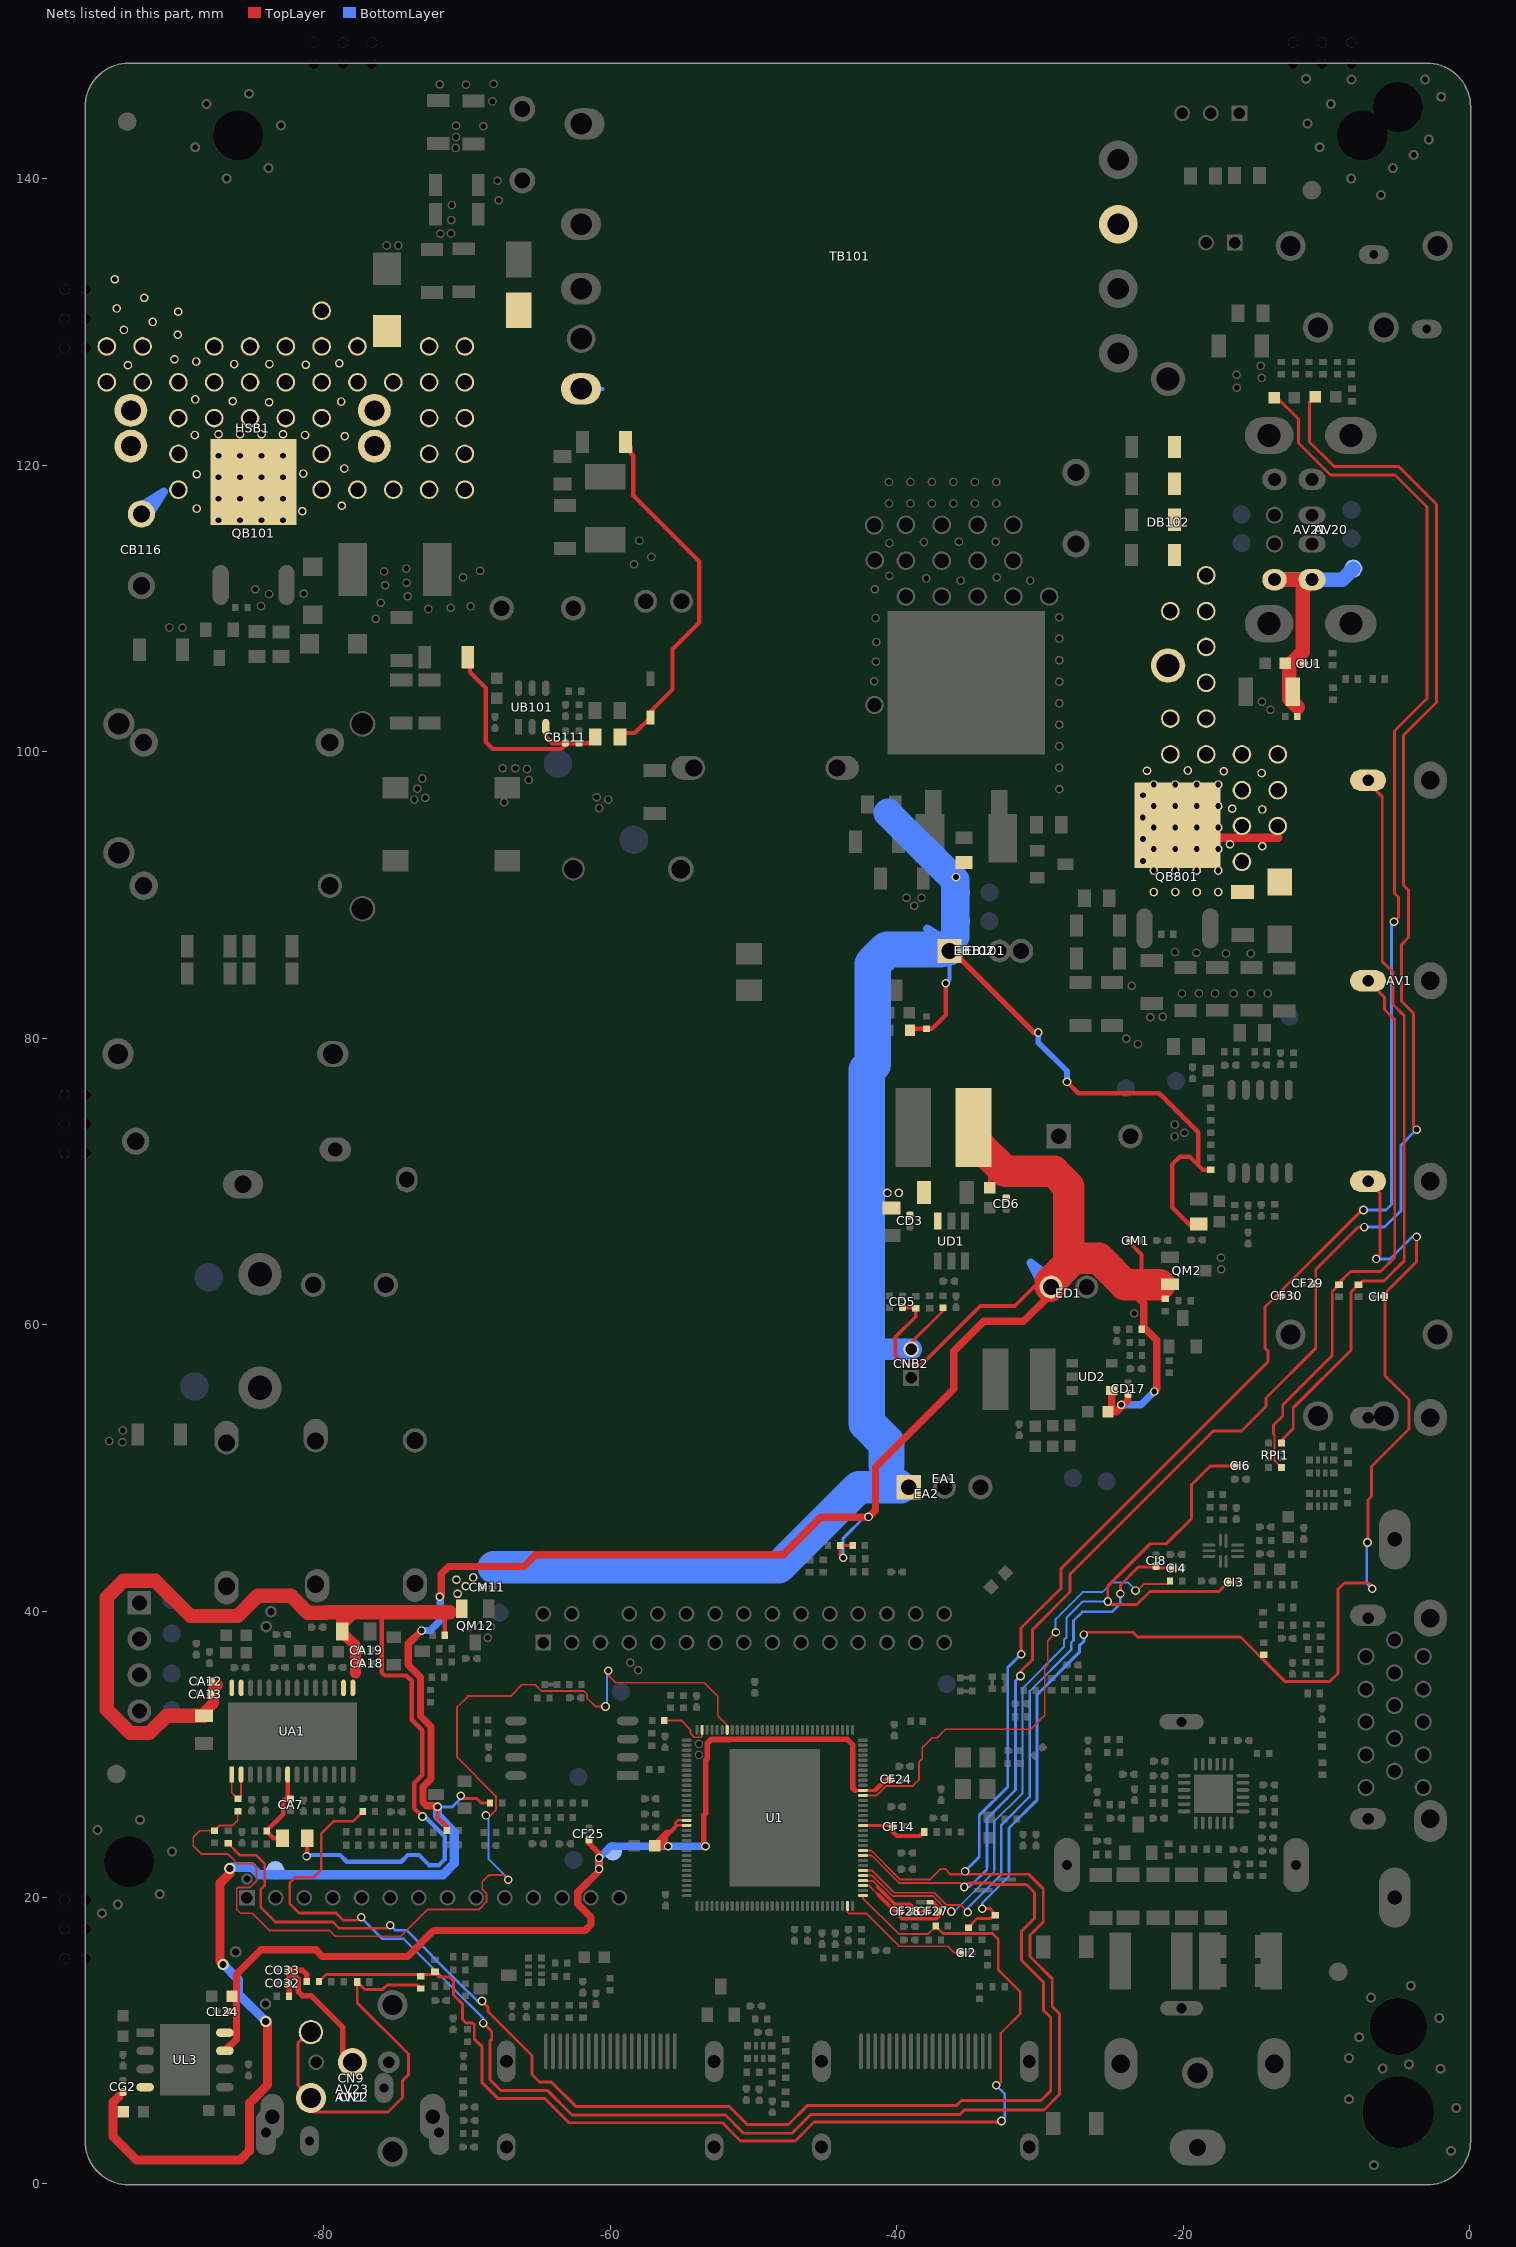
[diagram p0: the nets of this part, all layers, seen from the top]
# Altium PCB MISC86372.PcbDoc (part 7 of 16)
Units mm, origin at the board's own origin, x right, y up, seen from the top; angles counter-clockwise.
Board outline 96.73 x 148.13 mm, 2 copper layers (TopLayer, BottomLayer), stack 1.571 mm thick; 578 components, 318 nets, 2702 pads, 836 vias.

## Via types
v1: diameter 0.6, hole 0.4, TopLayer to BottomLayer, tented both sides, 816 vias
v2: diameter 0.7, hole 0.5, TopLayer to BottomLayer, tented both sides, 15 vias
v3: diameter 0.8, hole 0.5, TopLayer to BottomLayer, tented both sides, 5 vias

## Nets (pads, with @x,y where several pads share a name; then routed paths per layer and width w, separated by ;. In a path a pad name is that pad's centre, name@x,y a point inside that pad or via, vN(x,y) a via of type N, cw(c..) or ccw(c..) an arc to the next point about the centre after c; other vN are vias at no path point) (continued)
5V_STB: 5V_STB.1 CD5.2@-39.603,61.164 CD5.2@-39.603,61.339 CD6.2@-32.36,68.87 CD6.2@-32.36,68.695 CD7.2 CD16.2 CD17.2@-23.849,55.1 CD17.2@-23.849,55.275 CG1.2 CG2.2@-94.027,6.377 CG2.2@-94.027,6.552 CM1.2@-23.556,65.863 CM1.2@-23.731,65.863 ED1.1 LD1.2 pad.VIA5@-22.022,55.321 pad.VIA5@-24.337,54.392 pad.VIA5@-71.907,40.996 pad.VIA5@-73.177,38.633 pad.VIA5@-84.051,11.354 pad.VIA5@-86.563,22.022 pad.VIA5@-87.027,15.327 QM2.S RD3.2 RD7.2 RF8.2 RF9.2 RK1.2 RK5.1 RM3.2 UD2.4 UL3.4 | length 202.9
  TopLayer w0.203: v1(-70.434,27.102) v1@-70.258,26.925 ; v1@-70.423,26.925 v1@-70.258,26.925 ; RK1.2@-68.503,26.702 RK1.2@-68.395,26.594 -69.005,26.594 -69.337,26.925 v1@-70.258,26.925 ; v1(-43.741,43.715) -43.949,43.923 RF9.2@-43.949,44.564 RF8.2@-43.072,44.564
  TopLayer w0.254: CD5.2@-39.603,61.164 -38.702,61.164 RD3.2@-38.677,61.139 -38.677,60.545 -40.083,59.139 -40.083,57.826 -39.449,57.191 -38.268,57.191 -34.168,61.29 -31.766,61.29 -30.372,62.684 ED1.1@-29.293,62.684 ; CD7.2@-33.503,69.551 -33.503,70.841 ; CM1.2@-23.731,65.863 -23.731,65.706 -22.918,64.893 -22.918,62.789
  TopLayer w0.305: v1(-72.063,26.338) -72.063,25.577 -71.418,24.932 RK5.1@-71.418,24.669
  TopLayer w0.381: -23.849,54.736 CD17.2@-23.849,55.1
  TopLayer w0.508: pad.VIA5@-73.177,38.633 -74.1,37.711 -74.1,36.228 -73.254,35.382 -73.254,32.664 -72.517,31.928 -72.517,28.296 ; -73,27.813 -72.517,28.296 ; v1(-72.063,26.338) -72.135,26.41 -72.835,26.41 -73.068,26.643 -73.068,27.738 -72.517,28.289 -72.517,28.296 ; pad.VIA5@-71.797,40.996 -71.797,42.59 -71.283,43.104 -66.026,43.104 -65.197,43.933 -47.916,43.933 -45.3,46.549 -41.973,46.549 -41.478,47.044 -41.478,50.037 -36.018,55.497 -36.018,58.14 -33.934,60.223 -31.153,60.223 -29.293,62.084 ED1.1@-29.293,62.684 ; UD2.4@-24.99,55.393 -24.99,54.015 -25.102,53.904 -24.682,53.904 -23.849,54.736 ; -24.067,62.789 -22.766,61.488 -22.766,59.816 -21.844,58.894 -21.844,55.499 pad.VIA5@-22.022,55.321 ; -21.858,62.569 -21.638,62.789
  TopLayer w0.635: -94.289,6.121 -94.704,5.706 -94.704,3.309 -93.083,1.688 -88.4,1.688 -88.388,1.676 -85.827,1.676 -85.194,2.309 -85.194,5.635 -84.903,5.927 -84.903,5.932 -83.922,6.913 -83.922,11.225 pad.VIA5@-84.051,11.354 ; pad.VIA5@-87.027,15.327 -87.244,15.544 -87.244,20.993 -86.563,21.674 pad.VIA5@-86.563,22.022
  TopLayer w2.2: LD1.2@-34.154,72.425 -32.417,70.688 -29.056,70.688 -27.983,69.615 -27.983,64.263 ; ED1.1@-29.293,62.684 -29.293,62.953 -27.983,64.263 ; -21.638,62.789 -22.918,62.789 -24.067,62.789 -25.899,64.621 -27.625,64.621 -27.983,64.263
  BottomLayer w0.203: v1(-72.063,26.338) -72.037,26.313 -71.036,26.313 v1@-70.423,26.925 ; v1(-43.741,43.715) -43.741,45.082 -42.254,46.569 v1(-41.973,46.569)
  BottomLayer w0.508: pad.VIA5@-73.177,38.633 -72.568,38.633 -71.861,39.341 -71.861,40.996 pad.VIA5@-71.857,40.996 ; ED1.1@-29.228,62.619 ED1.1@-29.228,63.239 ; pad.VIA5@-24.337,54.392 -22.951,54.392 pad.VIA5@-22.022,55.321
  BottomLayer w0.635: pad.VIA5@-87.027,15.327 -85.954,14.254 -85.954,13.257 pad.VIA5@-84.051,11.354 ; pad.VIA5@-86.563,22.022 -86.476,22.109 -85.025,22.109 -84.506,21.59 -71.679,21.59 -70.891,22.377 -70.891,24.551 -72.063,25.723 v1(-72.063,26.338)
5V_USB2.0: 5V.1 AV20.1@-11.01,112 AV21.1 AV21.5 CU1.1 CU2.1 FU1.1 RU4.1 | length 18.3
  TopLayer w1.016: AV21.1@-13.63,112 AV21.5@-11.01,112 -11.665,111.345 -11.665,106.979 -12.598,106.046 -12.598,103.695 -12.002,103.099
  BottomLayer w1.016: AV21.1@-13.63,112 AV21.5@-11.01,112 -8.904,112 5V.1@-8.128,112.776
12V: CA1.2 CA2.2 CA12.2@-87.818,35.105 CA12.2@-87.993,35.105 CA13.2@-87.843,34.188 CA13.2@-88.018,34.188 CA18.2@-77.42,36.347 CA18.2@-77.245,36.347 CA19.2@-77.45,37.272 CA19.2@-77.275,37.272 CD1.2 CD2.1 CD3.2@-39.079,67.481 CD3.2@-39.079,67.656 CM11.2@-68.845,41.652 CM11.2@-69.02,41.652 CNB2.2 EA1.1 EA2.1 EB101.1@-36.323,86.081 EB102.1@-36.323,86.081 pad.VIA5@-35.865,91.237 pad.VIA5@-39.853,69.19 pad.VIA5@-40.654,69.19 pad.VIA5@-69.571,42.342 pad.VIA5@-70.098,41.732 pad.VIA5@-70.663,41.199 pad.VIA5@-70.739,42.189 QM12.S RA25.1 RB131.2 RB135.1 RB139.1 RB140.1 RB816.1 RD1.1 RM13.1 TB101.9 TP_12VA+.1 TP_12VB+.1 UA1.15 UA1.16 UA1.27 UA1.28 UD1.3 | length 213.5
  TopLayer w0.203: CNB2.2@-39,58.275 -39,58.733 -36.779,60.954 RD1.1@-36.779,61.157
  TopLayer w0.3: RB131.2@-39.122,80.442 -38.908,80.656 RB139.1@-37.922,80.656 -37.534,80.656 -36.576,81.614 v1(-36.576,83.82) ; EB102.1@-36.323,86.081 EB102.1@-36.115,86.081 ; v1(-28.118,76.937) -27.33,76.149 -21.675,76.149 -18.948,73.423 -18.948,71.305 ; RB816.1@-19.025,66.876 -19.47,66.876 -20.777,68.183 -20.777,71.171 -20.244,71.704 -19.538,71.704 -18.631,70.797 RB135.1@-18.085,70.797
  TopLayer w0.305: v1(-81.204,22.885) -81.153,22.936 RA25.1@-81.153,24.13 ; -75.963,39.885 -75.963,35.711 -75.755,35.503 -74.237,35.503 -73.863,35.129 -73.863,32.412 -73.127,31.675 -73.127,28.548 -73.677,27.997 -73.677,26.222 v1(-73.108,25.653) ; RM13.1@-71.55,38.278 RM13.1@-71.55,38.303 -71.55,39.497
  TopLayer w0.4: EB102.1@-36.115,86.081 -30.425,80.391 v1(-30.124,80.391)
  TopLayer w0.762: CA1.2@-88.361,32.913 -87.69,33.584 -87.69,34.575 -87.417,34.848 ; CA2.2@-78.715,38.583 -78.715,38.509 -77.785,37.579 -77.785,35.687
  TopLayer w1: CA1.2@-88.367,32.691 -90.973,32.691 -92.179,31.485 -93.51,31.485 -95.148,33.123 -95.148,40.947 -93.994,42.102 -91.76,42.102 -89.312,39.654 -86.007,39.654 -84.603,41.057 -82.319,41.057
  TopLayer w1.016: -82.256,41.021 -81.115,39.881 -79.822,39.881 ; -79.784,39.919 -71.207,39.919 ; -78.646,39.276 -78.033,39.889
  BottomLayer w0.3: v1(-36.576,83.82) -36.323,84.073 EB102.1@-36.323,86.081
  BottomLayer w0.305: v1(-81.204,22.885) -81.125,22.965 -78.87,22.965 -78.397,22.492 -74.6,22.492 -74.127,22.965 -73.358,22.965 -72.657,22.263 -71.958,22.263 -71.564,22.656 -71.564,24.273 -72.945,25.653 v1(-73.108,25.653)
  BottomLayer w0.4: v1(-30.124,80.391) -30.124,79.699 -28.118,77.693 v1(-28.118,76.937)
  BottomLayer w1.524: -41.453,58.217 -41.395,58.275 CNB2.2@-39,58.275
  BottomLayer w2: -40.615,95.707 -35.916,91.008 -35.916,87.071 -36.323,86.664 EB102.1@-36.323,86.081
  BottomLayer w2.286: -68.117,43.054 -48.248,43.054 -42.658,48.643 -39.742,48.643 EA1.1@-39.714,48.643
  BottomLayer w2.54: -40.714,50.199 -40.714,51.737 -42.089,53.113 -42.089,77.767 -41.686,78.171 -41.686,85.172 -40.672,86.186 EB102.1@-36.972,86.186
12V_OVP: DB107.A RB113.2 RB114.2 TB101.6 | length 27.4
  TopLayer w0.3: TB101.6@-62.562,124.796 TB101.6@-62.038,125.319 ; RB113.2@-59.319,101.295 -58.42,101.295 -58.289,101.295 DB107.A@-57.201,102.384 -57.201,102.79 -55.651,104.339 -55.651,107.137 -53.797,108.992 -53.797,113.284 -58.395,117.881 -58.395,120.65 -58.572,120.828 -58.572,121.286 RB114.2@-58.825,121.539
  BottomLayer w0.3: TB101.6@-62.038,125.319 -60.549,125.319
+1.8V_DDR: +1.8V_DDR.1 CF3.2 CF24.1 CF25.1 CL23.1 CL24.2@-86.64,12.038 CL24.2@-86.815,12.038 pad.VIA5@-60.782,21.996 pad.VIA5@-60.782,22.764 U1.54 U1.113 U1.114 UL3.7 UL3.8 | length 79.2
  TopLayer w0.178: U1.114@-54.663,25.031 -55.296,25.031 -55.456,24.87 -55.456,25.214 -55.29,25.381 U1.113@-54.663,25.381
  TopLayer w0.203: -42.908,27.481 -41.583,27.481
  TopLayer w0.305: -56.058,24.308 -56.058,24.325 -55.484,24.899 ; -41.497,27.481 -40.732,28.245 CF24.1@-40.455,28.245
  TopLayer w0.381: CF25.1@-61.493,24.01 -61.493,23.791 -61.062,23.359 -60.782,23.08 -60.782,23.044 pad.VIA5@-60.782,22.764 ; v1(-53.354,23.578) -53.463,23.687 -53.463,25.748 -53.336,25.875 -53.336,29.591 -53.219,29.709 -53.219,30.779 -53.025,30.973 ; -53.193,30.779 -52.999,30.973 ; -51.664,31.027 -52.945,31.027 ; -42.908,27.481 -43.081,27.654 -43.081,30.679 -43.442,31.04 -52.933,31.04 -52.945,31.027 ; -53.025,30.973 -52.999,30.973 ; -53.025,30.973 -52.971,31.027 -52.945,31.027 ; -52.999,30.973 -52.945,31.027
  TopLayer w0.508: UL3.7@-86.906,9.295 -86.098,10.103 -86.098,14.636 -84.389,16.345 -80.56,16.345 -80.103,15.888 -74.13,15.888 -72.314,17.704 -61.758,17.704 -61.341,18.12 -61.341,18.623 -62.27,19.552 -62.27,20.365 -60.782,21.853 pad.VIA5@-60.782,21.996 pad.VIA5@-60.782,22.764 ; CF3.2@-56.908,23.628 CF3.2@-56.886,23.628 ; -56.145,24.304 -56.21,24.304 ; -56.036,24.478 -56.21,24.304 ; v1(-55.965,23.578) v1@-56.014,23.628 ; CF3.2@-56.886,23.628 v1@-56.014,23.628 ; CF3.2@-56.886,23.628 -56.21,24.304 ; -56.21,24.304 -56.21,23.823 v1@-56.014,23.628
  BottomLayer w0.508: pad.VIA5@-60.782,21.996 pad.VIA5@-60.782,22.764 -59.968,23.578 v1(-55.965,23.578) v1(-53.354,23.578)
AMP_L_OUT_IC: CA32.2 CF29.1 RA3.1 U1.41 | length 225.5
  TopLayer w0.127: U1.41@-42.362,22.931 -41.756,22.931 -39.844,21.018 -35.574,21.018 v1(-35.286,20.731)
  TopLayer w0.178: RA3.1@-86.535,23.797 -86.704,23.797 -85.843,22.936 -84.712,22.936 -84.138,22.362 -84.138,20.841 -84.391,20.587 -84.391,19.305 -83.374,18.288 -79.366,18.288 -78.922,17.843 -75.578,17.843
  TopLayer w0.203: v1@-68.956,12.764 -68.527,12.335 -68.527,12.038 -65.456,8.967 -65.456,7.646 -64.934,7.125 -64.12,7.125 -62.415,5.42 -51.702,5.42 -50.436,4.153 -47.564,4.153 -46.252,5.466 -35.853,5.466 -35.487,5.831 -29.932,5.831 -29.252,6.511 -29.252,11.63 -29.753,12.13 -29.753,14.077 -31.305,15.63 -31.305,17.625 -30.383,18.547 -30.383,20.353 -30.939,20.909 -33.284,20.909 -33.385,21.011 -35.006,21.011 v1(-35.286,20.731) ; v1(-31.361,35.464) -31.361,35.772 -30.51,36.623 -30.51,38.719 -27.902,41.327 -27.902,42.572 -17.908,52.565 -15.939,52.565 -14.224,54.281 -14.224,54.873 -10.747,58.35 -10.747,63.834 -7.778,66.802 v1(-7.366,66.802) ; CA32.2@-10.769,124.765 -11.176,124.358 -11.176,121.616 -9.473,119.913 -4.967,119.913 -2.324,117.27 -2.324,103.433 -4.637,101.12 -4.637,90.692 -4.267,90.322 -4.267,87.014 -4.775,86.506 -4.775,82.583 -3.912,81.719 -3.912,73.812 v1(-3.708,73.609)
  BottomLayer w0.152: v1(-35.286,20.731) -34.932,20.731 -33.706,21.957 -33.706,22.086
  BottomLayer w0.178: v1(-75.362,18.059) -75.024,17.721 -74.237,17.721 -70.663,14.148 -69.279,12.764
  BottomLayer w0.203: -33.706,22.086 -33.706,25.514 -31.72,27.5 -31.72,35.117 v1@-31.372,35.464 ; v1(-7.366,66.802) -5.944,66.802 -4.801,67.945 -4.801,72.517 v1(-3.708,73.609)
  other v1: -68.956,12.775
AMP_MUTE_OUT: RA2.1 UA1.1 UA1.2 | length 3.7
  TopLayer w0.127: UA1.1@-86.422,28.611 -86.422,28.561 -86.422,27.304 RA2.1@-86.001,26.883 -85.772,27.113 UA1.2@-85.772,28.561
AMP_MUTE_OUT_IC: RA1.1 RA2.2 U1.90 | length 75.6
  TopLayer w0.127: -88.648,24.657 -89.114,24.191 -89.114,23.614 -88.544,23.044 -86.705,23.044 -86.026,22.365 -84.949,22.365 -84.709,22.125 -84.709,21.146 -85.15,20.705 -85.983,20.705 -86.08,20.608 -86.08,19.16 -85.817,18.898 -85,18.898 -83.807,17.704 -79.608,17.704 -79.202,17.297 -74.628,17.297 -72.774,19.152 -69.191,19.152 -68.649,19.694 -68.649,20.286 -68.936,20.572 -68.936,21.094 -68.452,21.578 -67.475,21.578 v1(-67.132,21.234) ; -88.609,24.661 RA1.1@-87.641,24.661 -87.264,25.037 -86.359,25.037 -86.001,25.395 RA2.2@-86.001,26.033 ; -68.351,25.73 -67.982,26.1 -67.982,27.08 -70.691,29.789 -70.691,33.301 -69.93,34.061 -66.959,34.061 -66.172,34.849 -65.247,34.849 -64.815,34.417 -61.848,34.417 -61.624,34.193 -61.624,33.912 -61.054,33.342 v1@-60.331,33.342 ; -60.143,35.502 -59.632,34.992 -53.437,34.992 -52.807,34.361 -52.495,34.049 -52.495,32.694 -51.838,32.038 U1.90@-51.838,31.707 U1.90@-51.838,31.656
  BottomLayer w0.127: v1(-68.682,25.73) -68.499,25.548 -68.499,22.682 v1@-67.132,21.315 ; v1@-60.236,33.427 v1@-60.236,35.732
  other v1: -60.331,33.333 -60.143,35.825
AMP_R_OUT_IC: CA31.2 CF30.1 RA14.1 U1.42 | length 228.2
  TopLayer w0.127: U1.42@-42.362,23.281 -41.782,23.281 -39.749,21.247 -37.691,21.247 -36.942,21.996 -36.629,21.996 -36.253,21.62
  TopLayer w0.178: -77.61,18.402 -78.619,18.402 -79.135,18.919 -81.736,18.919 -82.385,19.567 -82.385,21.008 -81.967,21.426 -80.696,21.426 -80.162,21.96 -80.162,24.463 -79.311,25.315 -77.968,25.315 RA14.1@-77.274,26.01
  TopLayer w0.203: v1(-68.864,11.233) -68.275,10.644 -68.275,10.108 -68.408,9.976 -68.408,7.286 -67.637,6.515 -64.372,6.515 -62.667,4.81 -51.955,4.81 -50.83,3.685 -50.83,3.681 -50.692,3.543 -47.312,3.543 -45.999,4.856 -35.601,4.856 -35.286,5.171 -29.73,5.171 -28.643,6.258 -28.643,11.882 -29.143,12.382 -29.143,14.329 -30.696,15.882 -30.696,17.372 -30.425,17.643 -29.774,18.294 -29.774,20.606 -30.788,21.62 -36.253,21.62 ; v1(-31.318,36.982) -31.318,38.811 -28.538,41.592 -28.538,42.952 -14.097,57.393 -14.097,58.145 -14.3,58.347 -14.3,61.215 v1@-7.569,67.945 ; CA31.2@-13.561,124.813 -11.963,123.215 -11.963,121.541 -9.726,119.304 -5.22,119.304 -2.984,117.069 -2.984,103.706 -5.246,101.444 -5.246,90.108 -4.978,89.84 -4.978,88.417 v1@-5.246,88.15
  BottomLayer w0.178: v1(-77.394,18.618) -75.887,17.112 -74.417,17.112 -70.895,13.589 -68.864,11.559 v1(-68.864,11.233)
  BottomLayer w0.203: v1(-35.23,21.819) -35.23,21.833 -34.239,22.824 -34.239,25.735 -32.253,27.721 -32.253,36.048 v1(-31.318,36.982) ; v1(-7.417,67.996) -5.853,67.996 -5.461,68.387 -5.461,87.935 v1(-5.283,88.113)
AU_CTRL_IC: RI3.1 U1.53 | length 33.4
  TopLayer w0.127: U1.53@-42.363,27.131 -41.398,27.131 -40.741,27.788 -38.869,27.788 -38.438,28.219 -38.438,29.471 -38.226,29.683 -38.226,30.462 -37.531,31.157 -37.182,31.157 -36.598,31.741 -30.633,31.741 -29.665,32.709 -29.665,36.014 -29.464,36.215 -29.464,37.938 v1(-28.888,38.514) ; v1@-23.343,41.286 v1@-23.204,41.425 ; v1@-23.335,41.207 -23.292,41.25 v1@-23.292,41.286 ; v1(-23.335,41.425) v1@-23.204,41.425 ; RI3.1@-20.974,42.139 RI3.1@-20.923,42.088 -21.118,41.892 -22.736,41.892 v1@-23.204,41.425
  BottomLayer w0.127: v1(-28.888,38.514) -28.909,38.536 -28.909,39.435 -27.023,41.322 -25.689,41.322 ; -25.639,41.322 -24.974,41.986 -23.84,41.986 -23.335,41.481 v1(-23.335,41.425) v1@-23.335,41.207
AUVAG: CF27.2@-37.734,19.043 CF27.2@-37.909,19.043 CF28.2@-38.934,19.039 CF28.2@-39.109,19.039 U1.36 | length 5.6
  TopLayer w0.127: U1.36@-42.341,21.158 -41.667,21.158 -41.268,20.76 -41.268,20.673
  TopLayer w0.254: -41.311,20.716 -41.268,20.673 -40.127,19.533 -39.065,19.533 -38.934,19.401 CF28.2@-38.934,19.039 -37.913,19.039 CF27.2@-37.909,19.043
AUVRM: CF27.1 CF28.1 LF6.JP_1K U1.35 | length 7.9
  TopLayer w0.127: U1.35@-42.362,20.831 -41.924,20.831 -41.232,20.139
  TopLayer w0.254: -41.304,20.207 -40.224,19.126 ; -40.137,19.039 CF28.1@-39.784,19.039 -39.791,19.032 -39.791,18.658 -39.643,18.51 -37.218,18.51 -37.059,18.669 CF27.1@-37.059,19.043 -37.059,19.274 -37.444,19.66 LF6.JP_1K@-37.678,19.66
AV1_CVBS_IN_IC: CI2.2@-35.404,16.129 CI2.2@-35.579,16.129 U1.31 | length 9.5
  TopLayer w0.127: U1.31@-43.438,19.406 -43.438,18.977 -43.334,18.872 -42.102,18.872 -40.394,17.165 -39.827,16.597 -36.452,16.597 -35.984,16.129 CI2.2@-35.579,16.129 ; CI2.2@-35.528,16.18 CI2.2@-35.477,16.129
AV1_L_IN_IC: CI3.1 CI6.1 RI5.2 U1.37 | length 59
  TopLayer w0.127: U1.37@-42.362,21.531 -41.712,21.531 -40.286,20.104 -37.475,20.104 -37.057,19.686 ; -36.669,19.297 -37.057,19.686 ; v1(-36.199,19.021) -36.392,19.021 -37.057,19.686
  TopLayer w0.203: v1@-25.273,40.462 v1(-25.273,40.665) -25.273,41.724 -22.303,44.694 -21.184,44.694 -19.431,46.446 -19.431,48.815 -18.12,50.126 -17.927,50.126 CI6.1@-16.432,50.126 ; v1@-25.26,40.45 -23.24,40.45 -22.317,41.372 -17.517,41.372 CI3.1@-16.896,41.993
  BottomLayer w0.127: v1(-36.199,19.021) -35.977,19.021 -33.198,21.8 -33.198,21.92 -33.189,21.92
  BottomLayer w0.152: -33.189,21.92 -33.189,25.312 -31.353,27.149 -31.212,27.29 -31.212,34.614 -28.321,37.505 -28.321,37.991 -28.156,38.156 -28.156,39.524 -27.015,40.665 v1@-25.324,40.665
AV1_R_IN_IC: CI4.1 CI8.1 RI6.2 U1.38 | length 41.4
  TopLayer w0.127: U1.38@-42.363,21.881 -41.712,21.881 -40.164,20.333 -37.381,20.333 -36.534,19.486 -35.545,19.486 v1@-34.982,18.922
  TopLayer w0.203: v1(-24.384,41.207) -24.384,41.823 -23.121,43.085 CI8.1@-21.895,43.085 ; CI8.1@-21.895,42.996 RI6.2@-20.921,42.996
  BottomLayer w0.152: v1(-35.038,18.97) -35.038,19.286 -34.982,19.343 ; v1@-34.982,18.922 -34.982,19.343 ; -32.694,21.768 -32.694,21.631 -34.982,19.343
  BottomLayer w0.178: -32.694,21.768 -32.694,25.067 -30.716,27.045 -30.716,34.4 -27.826,37.29 -27.826,37.786 -27.661,37.951 -27.661,39.319 -27.033,39.946 -25.026,39.946 ; -24.975,39.946 -24.384,40.538 v1(-24.384,41.207)
AV_CVBS_IN: AV1.1 CI1.1 DI1.K RI1.2 RI2.2 | length 90.5
  TopLayer w0.203: RI2.2@-35,17.925 -34.4,18.524 -33.437,18.524 -33.122,18.84 -33.501,19.219 v1(-34.027,19.219) ; v1(-26.937,38.354) -26.771,38.52 -23.515,38.52 -23.184,38.189 -16.01,38.189 -12.914,35.093 -9.745,35.093 -9.195,35.643 -9.195,41.518 -8.752,41.961 -7.036,41.961 -6.807,41.732 v1(-6.807,41.554) ; v1@-7.105,44.939 -7.105,47.759 -6.858,48.006 -6.858,50.084 -4.242,52.701 -4.242,54.762 -5.925,56.446 CI1.1@-5.925,61.951 ; AV1.1@-7.1,70 -6.268,69.168 -6.268,65.938 ; v1(-6.524,64.581) -6.268,64.838 -6.268,65.938 ; -6.268,65.716 -6.268,65.938 ; CI1.1@-6.1,61.951 -6.1,61.995 -3.708,64.387 v1(-3.708,66.116)
  BottomLayer w0.152: v1(-34.027,19.219) -34.027,19.615 -32.173,21.469 -32.173,21.819
  BottomLayer w0.203: -32.173,21.819 -32.173,24.851 -30.196,26.829 -30.196,34.175 -27.254,37.116 -27.254,37.577 -26.937,37.894 v1(-26.937,38.354) ; v1@-7.191,44.78 -7.191,41.938 v1(-6.807,41.554) ; v1(-6.524,64.581) -5.557,64.581 -4.022,66.116 v1(-3.708,66.116)
  other v1: -7.137,44.78
AV_L_IN: AV1.3 DI2.K RPI1.1 | length 39.7
  TopLayer w0.127: -13.691,52.375 -13.624,52.308 -13.624,50.478 RPI1.1@-13.172,50.026
  TopLayer w0.203: -13.691,52.375 -13.691,52.984 -13.056,53.619 -13.056,54.385 -9.597,57.844 -9.597,58.018 -9.597,62.304 DI2.K@-9.119,62.782 ; DI2.K@-9.246,62.782 -8.328,63.7 -6.227,63.7 -5.232,64.695 -5.232,81.28 -5.944,81.991 -5.944,82.844 AV1.3@-7.1,84
AV_R_IN: AV1.5 DI3.K RPI1.7 | length 51.5
  TopLayer w0.203: -13.088,51.98 -12.319,52.749 -12.319,54.188 -8.276,58.231 -8.276,61.345 -8.276,62.278 DI3.K@-7.772,62.782 -7.512,63.043 -5.986,63.043 -4.572,64.457 -4.572,81.554 -5.359,82.341 -5.359,84.61 -6.104,85.355 -6.104,96.85 -7.1,97.846 AV1.5@-7.1,98
AVCC: CA7.2@-82.324,26.718 CA7.2@-82.324,26.893 RA8.1 RA25.2 UA1.7 | length 6.6
  TopLayer w0.305: RA25.2@-82.885,24.13 -83.508,24.13 -84.012,24.634 -82.828,25.818 -82.828,26.723 -82.657,26.893 CA7.2@-82.333,26.893 ; UA1.7@-82.522,28.611 -82.522,27.092 CA7.2@-82.333,26.903 ; CA7.2@-82.421,26.816 -82.344,26.893 CA7.2@-82.333,26.893 ; CA7.2@-82.387,26.809 CA7.2@-82.313,26.809 ; CA7.2@-82.333,26.968 CA7.2@-82.333,26.903 ; CA7.2@-82.303,26.893 CA7.2@-82.324,26.893 ; CA7.2@-82.333,26.893 CA7.2@-82.324,26.893 ; CA7.2@-82.333,26.893 CA7.2@-82.333,26.903 ; CA7.2@-82.333,26.903 CA7.2@-82.324,26.893
AVDD_DMPLL: CF14.2@-40.126,24.942 CF14.2@-40.301,24.942 L3.2 U1.47 | length 4.9
  TopLayer w0.203: U1.47@-42.362,25.031 CF14.2@-40.342,25.031
  TopLayer w0.305: CF14.2@-40.301,24.942 -40.301,24.591 -40.002,24.292 -38.388,24.292 L3.2@-38.068,24.613
AVOUT: CN9.4 CN9.5 DI9.K RO2.1 | length 28.4
  TopLayer w0.203: CN9.5@-81.053,10.6 -81.813,9.839 -81.813,6.913 CN9.4@-80.9,6 -80.9,5.208 -80.721,5.029 -75.513,5.029 -74.5,6.043 -74.5,7.212 -74.092,7.62 -74.092,9.068 -77.666,12.642 DI9.K@-77.666,14.101 -77.129,13.564 -75.915,13.564 -75.588,13.891 -75.082,13.891 ; -74.255,13.891 -75.082,13.891 ; RO2.1@-73.228,13.647 -73.473,13.891 -75.082,13.891
BRI_ADJ: RF29.1 U1.95 | length 3.7
  TopLayer w0.127: RF29.1@-56.217,32.36 -55.051,32.36 -54.407,31.715 -54.407,31.471 -54.127,31.191 -53.67,31.191 -53.588,31.273 U1.95@-53.588,31.707
BRO: CB111.2@-63.129,100.591 CB111.2@-63.129,100.766 RB104.2 RB113.1 RB142.1 UB101.3 | length 16.5
  TopLayer w0.3: RB142.1@-69.798,106.248 -69.798,105.541 -68.694,104.436 -68.694,100.66 -68.209,100.175 -63.414,100.175 -63.129,100.46 CB111.2@-63.129,100.591 RB104.2@-62.189,100.591 -61.473,100.591 RB113.1@-61.048,101.016 ; UB101.3@-64.506,101.85 UB101.3@-64.506,101.727 -64.506,101.031 -64.066,100.591 CB111.2@-63.291,100.591
COAX&CVBSOUT: AV22.1 AV23.2 CN1.1 CO32.1 CO33.2@-82.43,14.935 CO33.2@-82.605,14.935 RO3.1 RO33.2 | length 12.6
  TopLayer w0.381: CO32.1@-82.43,14.021 CO33.2@-82.43,14.935 ; RO33.2@-82.422,13.059 -82.402,13.079 CO32.1@-82.402,13.995 ; -81.788,14.053 -81.788,14.294 ; RO3.1@-81.187,14.129 -81.187,14.613 -81.509,14.935 CO33.2@-82.43,14.935 ; CN1.1@-78,8.5 -78.664,9.164 -78.664,10.928 -80.885,13.15 -81.5,13.15 -81.788,13.438 -81.788,14.294 ; CO33.2@-82.43,14.935 -81.788,14.294
CVBS_OUT_IC: DO1.K RO1.2 RO2.2 RO3.2 U1.33 | length 82.5
  TopLayer w0.127: U1.33@-42.362,20.131 -42.362,19.959 -39.862,17.459 -37.793,17.459 -37.28,17.971 RO1.2@-37.28,18.009
  TopLayer w0.178: RO1.2@-37.28,18.009 -36.759,17.487 -34.671,17.487 -33.308,17.487 -32.918,17.098 -32.918,14.962 -31.366,13.409 -31.366,11.898 -32.741,10.523 -32.741,7.112 v1@-32.959,6.893
  TopLayer w0.203: RO3.2@-80.337,14.129 -79.839,14.626 DO1.K@-72.111,14.626 ; DO1.K@-72.297,14.812 DO1.K@-72.111,14.626 ; -51.363,3.46 -50.913,3.01 -47.091,3.01 -45.778,4.323 -32.965,4.323 v1@-32.7,4.587 ; -51.363,3.464 -52.176,4.277 -62.888,4.277 -64.593,5.982 -67.858,5.982 -68.941,7.065 -68.941,9.577 -69.494,10.13 -69.494,11.125 -69.611,11.242 -70.068,11.242 -70.307,11.48 -70.307,12.543 -70.953,13.189 -70.953,14.187 -71.222,14.457 -71.941,14.457 DO1.K@-72.111,14.626
  BottomLayer w0.178: v1(-33.06,6.893) -32.452,6.286 -32.452,4.632 v1(-32.69,4.394)
D_QB101: BB101.1 CB116.1 DB106.A HSB1.1 HSB1.2 HSB1.3 HSB1.4 pad.VIA5@-70.149,118.283 pad.VIA5@-70.149,120.783 pad.VIA5@-70.149,123.283 pad.VIA5@-70.149,125.783 pad.VIA5@-70.149,128.283 pad.VIA5@-72.649,118.283 pad.VIA5@-72.649,120.783 pad.VIA5@-72.649,123.283 pad.VIA5@-72.649,125.783 pad.VIA5@-72.649,128.283 pad.VIA5@-75.149,118.283 pad.VIA5@-75.149,125.783 pad.VIA5@-77.649,118.283 pad.VIA5@-77.649,125.783 pad.VIA5@-77.649,128.283 pad.VIA5@-78.74,117.17 pad.VIA5@-78.537,122.022 pad.VIA5@-78.562,119.761 pad.VIA5@-78.791,124.435 pad.VIA5@-78.918,127.102 pad.VIA5@-80.149,118.283 pad.VIA5@-80.149,120.783 pad.VIA5@-80.149,123.283 pad.VIA5@-80.149,125.783 pad.VIA5@-80.149,128.283 pad.VIA5@-80.149,130.783 pad.VIA5@-81.255,127 pad.VIA5@-81.305,122.098 pad.VIA5@-81.432,119.405 pad.VIA5@-81.501,116.783 pad.VIA5@-82.649,123.283 pad.VIA5@-82.649,125.783 pad.VIA5@-82.649,128.283 pad.VIA5@-82.848,116.156 pad.VIA5@-82.848,117.656 pad.VIA5@-82.848,119.156 pad.VIA5@-82.848,120.656 pad.VIA5@-82.848,122.156 pad.VIA5@-83.82,124.384 pad.VIA5@-83.795,127.051 pad.VIA5@-84.348,116.156 pad.VIA5@-84.348,117.656 pad.VIA5@-84.348,119.156 pad.VIA5@-84.348,120.656 pad.VIA5@-84.348,122.156 pad.VIA5@-85.149,123.283 pad.VIA5@-85.149,125.783 pad.VIA5@-85.149,128.283 pad.VIA5@-85.848,116.156 pad.VIA5@-85.848,117.656 pad.VIA5@-85.848,119.156 pad.VIA5@-85.848,120.656 pad.VIA5@-85.848,122.156 pad.VIA5@-86.36,124.46 pad.VIA5@-86.258,127.051 pad.VIA5@-87.348,116.156 pad.VIA5@-87.348,117.656 pad.VIA5@-87.348,119.156 pad.VIA5@-87.348,120.656 pad.VIA5@-87.348,122.156 pad.VIA5@-87.649,123.283 pad.VIA5@-87.649,125.783 pad.VIA5@-87.649,128.283 pad.VIA5@-88.9,127.229 pad.VIA5@-88.875,116.967 pad.VIA5@-88.875,119.355 pad.VIA5@-88.976,124.587 pad.VIA5@-89,122.098 pad.VIA5@-90.17,130.708 pad.VIA5@-90.149,118.283 pad.VIA5@-90.149,120.783 pad.VIA5@-90.149,123.283 pad.VIA5@-90.149,125.783 pad.VIA5@-90.195,129.108 pad.VIA5@-90.424,127.381 pad.VIA5@-91.948,129.997 pad.VIA5@-92.532,131.674 pad.VIA5@-92.649,125.783 pad.VIA5@-92.649,128.283 pad.VIA5@-93.675,126.975 pad.VIA5@-93.955,129.438 pad.VIA5@-94.59,132.969 pad.VIA5@-94.463,130.937 pad.VIA5@-95.149,125.783 pad.VIA5@-95.149,128.283 QB101.D
D_QB801: CB129.1 DB102.K pad.VIA5@-13.4,94.804 pad.VIA5@-13.4,97.304 pad.VIA5@-13.4,99.804 pad.VIA5@-14.478,93.396 pad.VIA5@-14.478,95.961 pad.VIA5@-14.529,98.501 pad.VIA5@-15.9,92.304 pad.VIA5@-15.9,94.804 pad.VIA5@-15.9,97.304 pad.VIA5@-15.9,99.804 pad.VIA5@-16.586,96.012 pad.VIA5@-16.739,93.523 pad.VIA5@-17.17,98.628 pad.VIA5@-17.551,90.195 pad.VIA5@-17.551,91.695 pad.VIA5@-17.551,93.195 pad.VIA5@-17.551,94.695 pad.VIA5@-17.551,96.195 pad.VIA5@-17.551,97.695 pad.VIA5@-18.4,99.804 pad.VIA5@-18.4,102.304 pad.VIA5@-18.4,104.804 pad.VIA5@-18.4,107.304 pad.VIA5@-18.4,109.804 pad.VIA5@-18.4,112.304 pad.VIA5@-19.051,90.195 pad.VIA5@-19.051,91.695 pad.VIA5@-19.051,93.195 pad.VIA5@-19.051,94.695 pad.VIA5@-19.051,96.195 pad.VIA5@-19.051,97.695 pad.VIA5@-19.685,98.679 pad.VIA5@-20.9,99.804 pad.VIA5@-20.9,102.304 pad.VIA5@-20.9,109.804 pad.VIA5@-20.551,90.195 pad.VIA5@-20.551,91.695 pad.VIA5@-20.551,93.195 pad.VIA5@-20.551,94.695 pad.VIA5@-20.551,96.195 pad.VIA5@-20.551,97.695 pad.VIA5@-22.051,90.195 pad.VIA5@-22.051,91.695 pad.VIA5@-22.051,93.195 pad.VIA5@-22.051,94.695 pad.VIA5@-22.051,96.195 pad.VIA5@-22.051,97.695 pad.VIA5@-22.53,98.654 pad.VIA5@-22.809,92.354 pad.VIA5@-22.809,93.904 pad.VIA5@-22.809,96.952 pad.VIA5@-22.835,95.402 QB801.D RB124.1 RB125.1 RB126.1 RB136.1 ZDB801.K | length 4.5
  TopLayer w0.6: QB801.D@-17.86,93.981 -13.387,93.981